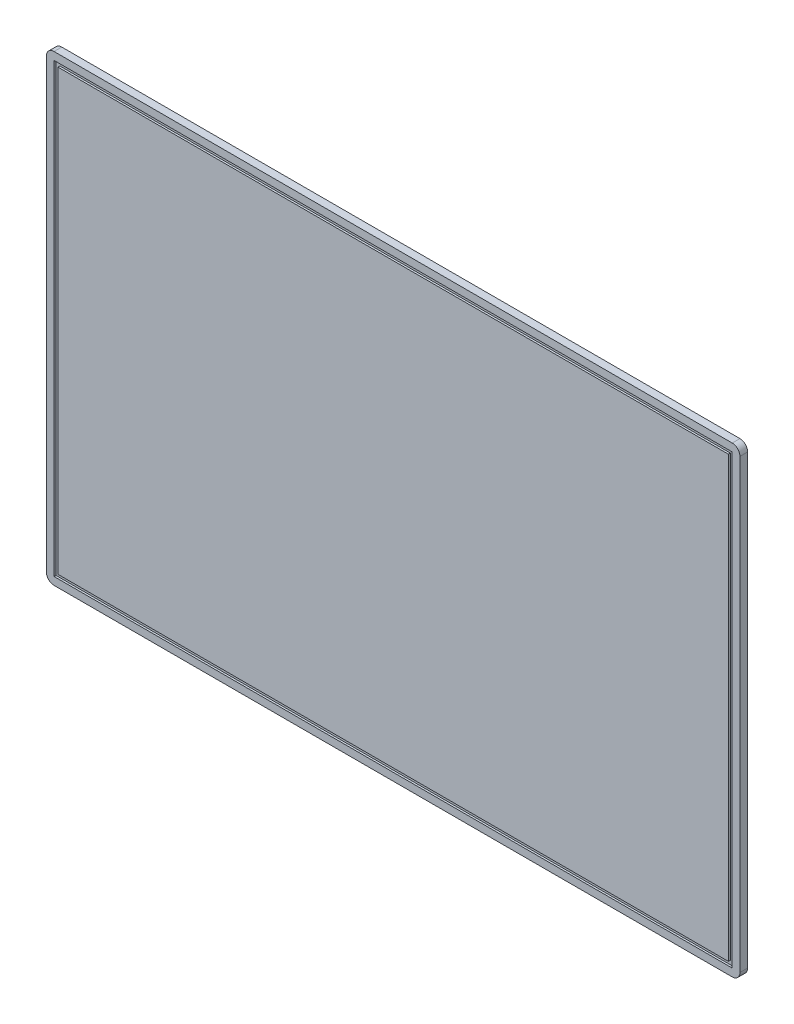
SolidWorks part; units mm, degrees
ref_plane "Front Plane" through (0, 0, 0) normal (0, 0, 1) x (1, 0, 0)
ref_plane "Top Plane" through (0, 0, 0) normal (0, 1, 0) x (1, 0, 0)
ref_plane "Right Plane" through (0, 0, 0) normal (1, 0, 0) x (0, 0, -1)
sketch "Sketch1" plane through (0, 0, 0) normal (0, 0, 1) x (1, 0, 0)
  line L1 (88, 60) -> (-88, 60)
  line L2 (90, 58) -> (90, -58)
  line L3 (88, -60) -> (-88, -60)
  line L4 (-90, 58) -> (-90, -58)
  line L5 (90, 60) -> (-90, -60) construction
  line L6 (90, -60) -> (-90, 60) construction
  arc A0 (88, 60) -> (90, 58) centre (88, 58) cw
  arc A1 (90, -58) -> (88, -60) centre (88, -58) cw
  arc A2 (-88, -60) -> (-90, -58) centre (-88, -58) cw
  arc A3 (-88, 60) -> (-90, 58) centre (-88, 58) ccw
  point P0 (0, 0)
  dimension "D3" = 2
  dimension "D1" = 180
  dimension "D2" = 120
extrude "Boss-Extrude1" add sketch "Sketch1" along normal blind 2
sketch "Sketch2" plane through (0, 0, 2) normal (0, 0, 1) x (1, 0, 0)
  line L0 (88, 60) -> (-88, 60) construction
  line L1 (88, 58) -> (-88, 58)
  line L2 (88, 58) -> (88, -58)
  line L3 (88, -58) -> (-88, -58)
  line L4 (-88, 58) -> (-88, -58)
  line L5 (88, 58) -> (-88, -58) construction
  line L6 (88, -58) -> (-88, 58) construction
  line L7 (-90, 58) -> (-90, -58) construction
  line L8 (87, 57) -> (-87, 57)
  line L9 (-87, 57) -> (-87, -57)
  line L10 (87, -57) -> (-87, -57)
  line L11 (87, 57) -> (87, -57)
  point P0 (0, 0)
  dimension "D1" = 2
  dimension "D2" = 2
  dimension "D3" = 1
extrude "Cut-Extrude1" cut sketch "Sketch2" against normal blind 0.5
